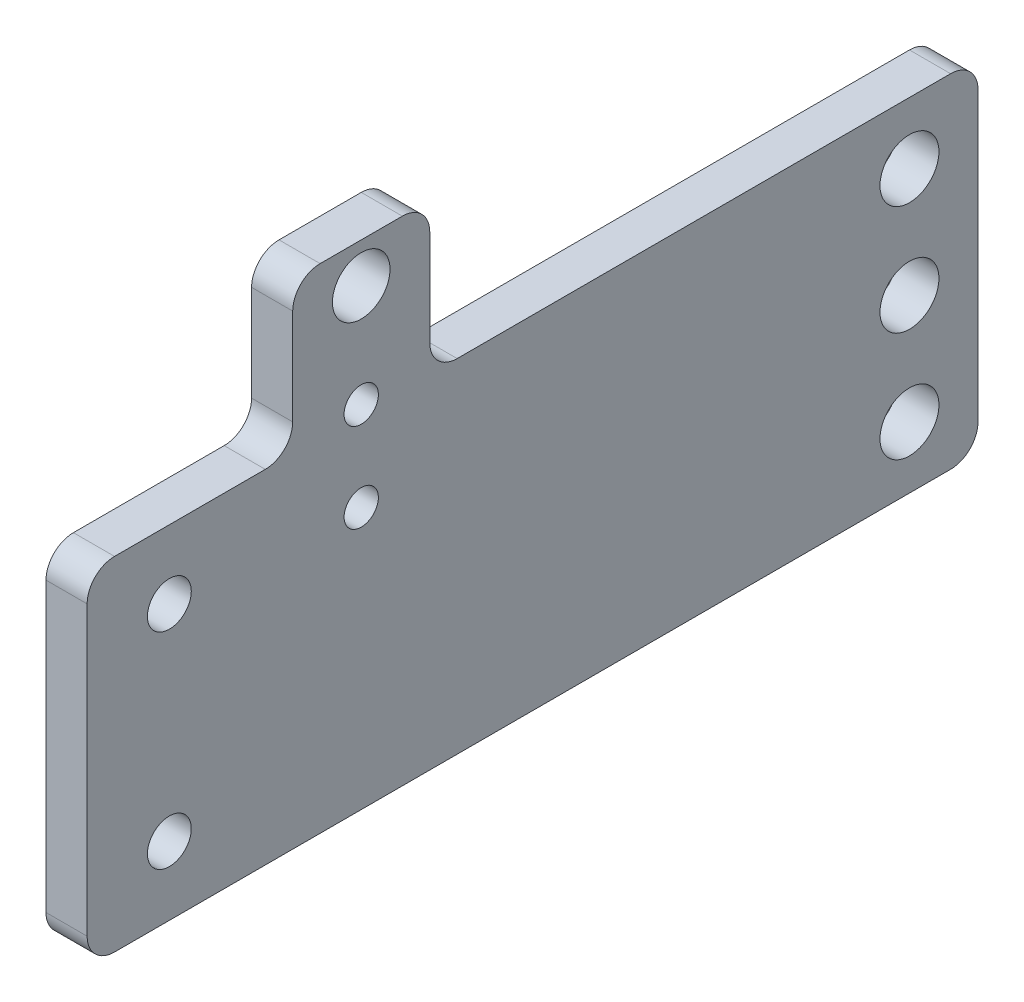
SolidWorks part; units mm, degrees
material "不锈钢201"
ref_plane "前视基准面" through (0, 0, 0) normal (0, 0, 1) x (1, 0, 0)
ref_plane "上视基准面" through (0, 0, 0) normal (0, 1, 0) x (1, 0, 0)
ref_plane "右视基准面" through (0, 0, 0) normal (1, 0, 0) x (0, 0, -1)
sketch "草图1" plane through (0, 0, 0) normal (1, 0, 0) x (0, 0, -1)
  line L0 (0, 0) -> (-38.0096, 0) construction
  line L1 (-32.5, 12.5) -> (32.5, 12.5)
  line L2 (-32.5, 12.5) -> (-32.5, -12.5)
  line L3 (-32.5, -12.5) -> (32.5, -12.5)
  line L4 (32.5, 12.5) -> (32.5, -12.5)
  line L5 (-32.5, 12.5) -> (32.5, -12.5) construction
  line L6 (-32.5, -12.5) -> (32.5, 12.5) construction
  circle A0 centre (-26.5, 7.5) radius 1.6
  circle A1 centre (-26.5, -7.5) radius 1.6
  point P0 (0, 0)
  dimension "D4" = 3.2
  dimension "D5" = 6
  dimension "D1" = 25
  dimension "D2" = 65
  dimension "D3" = 15
extrude "凸台-拉伸1" add sketch "草图1" along normal blind 3
fillet "圆角1" radius 2 4 edges at (1.5, -12.5, 32.5) (1.5, 12.5, 32.5) (1.5, -12.5, -32.5) (1.5, 12.5, -32.5)
hole_wizard "Ø4.3 (4.3) 直径孔1" positions "草图2" profile "草图3" hole size "Ø4.3" standard "GB"
sketch "草图2" plane through (0, 0, 0) normal (-1, 0, 0) x (0, 0, 1)
  line L0 (0, 0) -> (-35.503, 0) construction
  line L1 (-32.5, -10.5) -> (-32.5, 10.5) construction
  point P0 (-27.5, 8)
  point P8 (-27.5, -8)
  point P9 (-27.5, 0)
  dimension "D1" = 16
  dimension "D2" = 5
sketch "草图3" plane through (0, 8, -27.5) normal (0, 1, 0) x (0, 0, 1)
  line L0 (0, 0) -> (0, 12.7919)
  line L1 (0, 12.7919) -> (2.15, 11.5)
  line L2 (2.15, 11.5) -> (2.15, 0)
  line L5 (2.15, 0) -> (0, 0)
  line L10 (0, 12.7919) -> (-2.15, 11.5) construction
  line L11 (0, -6.35) -> (0, 107.95) construction
  dimension "孔直径" = 4.3
  dimension "孔深度" = 11.5
  dimension "导头角度" = 118
sketch "草图4" plane through (3, 0, 0) normal (1, 0, 0) x (0, 0, -1)
  line L1 (30.5, 12.5) -> (-30.5, 12.5) construction
  line L2 (-17.5, 23.5) -> (-7.5, 23.5)
  line L3 (-17.5, 23.5) -> (-17.5, 1.5)
  line L4 (-17.5, 1.5) -> (-7.5, 1.5)
  line L5 (-7.5, 23.5) -> (-7.5, 1.5)
  line L7 (-17.5, 23.5) -> (-7.5, 1.5) construction
  line L8 (-17.5, 1.5) -> (-7.5, 23.5) construction
  line L9 (32.5, -10.5) -> (32.5, 10.5) construction
  point P0 (-12.5, 12.5)
  dimension "D1" = 45
  dimension "D2" = 10
  dimension "D3" = 22
extrude "凸台-拉伸2" add sketch "草图4" against normal up to surface (3 mm away) up to face at (0, 8, -25.35)
sketch "草图5" plane through (0, 0, 0) normal (-1, 0, 0) x (0, 0, 1)
  line L0 (12.5, 23.5) -> (12.5, 1.4105) construction
  line L1 (17.5, 23.5) -> (7.5, 23.5) construction
  line L2 (17.5, 12.5) -> (30.5, 12.5) construction
  circle A0 centre (12.5, 20.6) radius 2.1
  dimension "D1" = 4.2
  dimension "D2" = 8.1
extrude "切除-拉伸1" cut sketch "草图5" against normal blind 10
fillet "圆角2" radius 2 4 edges at (1.5, 23.5, 17.5) (1.5, 23.5, 7.5) (1.5, 12.5, 7.5) (1.5, 12.5, 17.5)
hole_wizard "M3 螺纹孔1" positions "草图6" profile "草图8" tap size "M3" standard "GB"
sketch "草图6" plane through (0, 0, 0) normal (-1, 0, 0) x (0, 0, 1)
  point P0 (12.5, 6.6)
  point P3 (12.5, 13.1)
sketch "草图8" plane through (0, 6.6, 12.5) normal (0, 1, 0) x (0, 0, 1)
  line L0 (0, 0) -> (0, 9.2511)
  line L1 (0, 9.2511) -> (1.25, 8.5)
  line L2 (1.25, 8.5) -> (1.25, 0)
  line L5 (1.25, 0) -> (0, 0)
  line L10 (0, 9.2511) -> (-1.25, 8.5) construction
  line L11 (0, -6.35) -> (0, 107.95) construction
  dimension "螺纹孔钻头直径" = 2.5
  dimension "螺纹孔钻头深度" = 8.5
  dimension "导头角度" = 118
cosmetic thread "孔螺蚊线4" parameters "D1"=3, "D2"=3
cosmetic thread "孔螺蚊线5" parameters "D1"=3, "D2"=3
